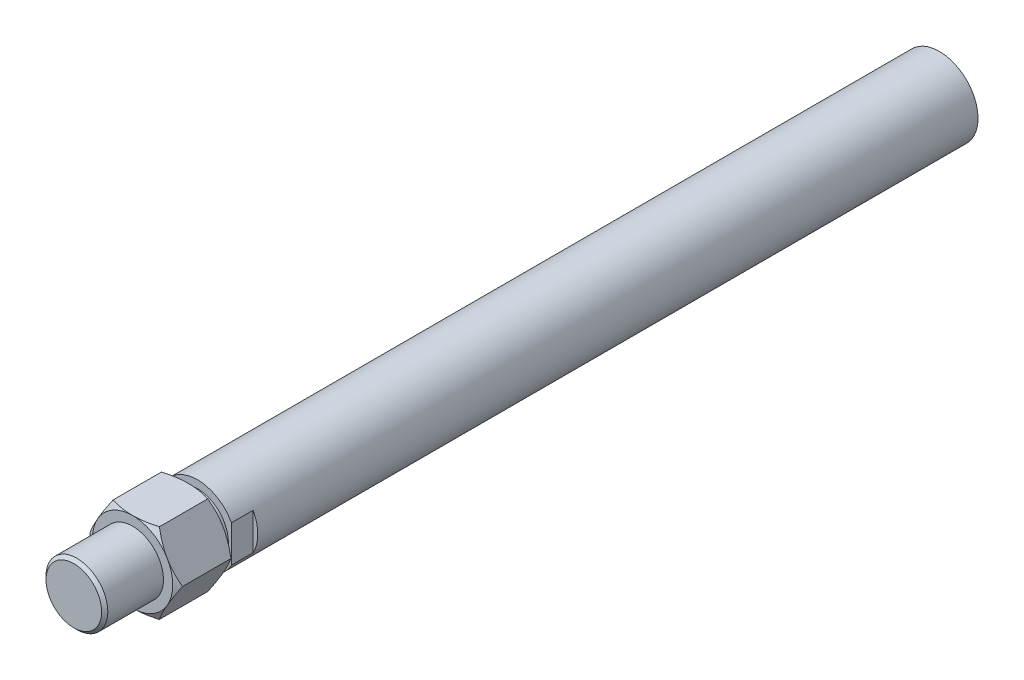
SolidWorks part; units mm, degrees
material "1.4000 (X6Cr13)"
ref_plane "Front Plane" through (0, 0, 0) normal (0, 0, 1) x (1, 0, 0)
ref_plane "Top Plane" through (0, 0, 0) normal (0, 1, 0) x (1, 0, 0)
ref_plane "Right Plane" through (0, 0, 0) normal (1, 0, 0) x (0, 0, -1)
sketch "Sketch1" plane through (0, 0, 0) normal (1, 0, 0) x (0, 0, -1)
  line L0 (0, 0) -> (-318, 0) construction
  line L1 (-243, 23.5) -> (0, 23.5)
  line L2 (0, 23.5) -> (0, -23.5)
  line L3 (0, -23.5) -> (-243, -23.5)
  line L24 (-243, 23.5) -> (-257, 23.5)
  line L25 (-257, 23.5) -> (-257, -23.5)
  line L26 (-257, 22.5208) -> (-264, 22.5208)
  line L27 (-264, 22.5208) -> (-264, -22.5208)
  line L28 (-264, 12.5) -> (-278, 12.5)
  line L29 (-278, 12.5) -> (-278, 10)
  line L30 (-278, 10) -> (-281, 10)
  line L31 (-318, 10) -> (-318, -10)
  line L32 (-278, -10) -> (-281, -10)
  line L33 (-264, -12.5) -> (-278, -12.5)
  line L34 (-257, -22.5208) -> (-264, -22.5208)
  line L35 (-243, -23.5) -> (-257, -23.5)
  line L38 (-299, 10) -> (-299, 15)
  line L39 (-299, 15) -> (-281, 15)
  line L40 (-281, 15) -> (-281, 10)
  line L41 (-281, -15) -> (-281, -10)
  line L42 (-299, -10) -> (-299, -15)
  line L43 (-299, -15) -> (-281, -15)
  line L44 (-299, 10) -> (-318, 10)
  line L45 (-299, -10) -> (-318, -10)
  line L46 (-278, -10) -> (-278, -12.5)
  point P4 (-60, 23.5)
  point P5 (-50, 23.5)
  point P6 (-38, 23.5)
  point P42 (-318, 0)
  point P44 (-318, 0)
  point P46 (-264, 0)
  point P48 (-257, 0)
  dimension "K" = 38
  dimension "RD" = 47
  dimension "KK" = 20
  dimension "VF" = 21
  dimension "WF" = 35
  dimension "D8" = 14
  dimension "S2" = 50
  dimension "S1" = 10
  dimension "A" = 40
  dimension "D14" = 45.0417
  dimension "螺母厚度" = 18
  dimension "D16" = 3
  dimension "螺母外径" = 30
  dimension "MM" = 25
  dimension "L1" = 183
sketch "Sketch3" plane through (0, 0, 0) normal (1, 0, 0) x (0, 0, -1)
  line L0 (-299, 10) -> (-318, 10) construction
  line L1 (-299, 15) -> (-281, 15) construction
  line L2 (-299, 10) -> (-299, 15) construction
  line L3 (-318, 10) -> (-318, -10) construction
  line L11 (-278, 10) -> (-281, 10) construction
  line L12 (-281, 15) -> (-281, 10) construction
  line L13 (-278, 12.5) -> (-278, 10) construction
  line L14 (-264, 12.5) -> (-278, 12.5) construction
  line L17 (-299, 10) -> (-318, 10)
  line L18 (-299, 15) -> (-281, 15)
  line L19 (-299, 10) -> (-299, 15)
  line L20 (-318, 10) -> (-318, 0)
  line L21 (-318, 0) -> (-38, 0)
  line L28 (-278, 10) -> (-281, 10)
  line L29 (-281, 15) -> (-281, 10)
  line L30 (-278, 12.5) -> (-278, 10)
  line L31 (-38, 12.5) -> (-278, 12.5)
  line L34 (-38, 12.5) -> (-38, 0)
  line L36 (0, 0) -> (-318, 0) construction
revolve "Revolve1" add sketch "Sketch3" angle 360 about L21
cosmetic thread "Cosmetic Thread1" parameters "D1"=38, "D2"=17
sketch "Sketch5" plane through (0, 0, 299) normal (0, 0, 1) x (1, 0, 0)
  line L0 (0, 0) -> (15, 0) construction
  line L1 (7.5, 12.9904) -> (-7.5, 12.9904)
  line L2 (-7.5, 12.9904) -> (-15, 0)
  line L3 (-15, 0) -> (-7.5, -12.9904)
  line L4 (-7.5, -12.9904) -> (7.5, -12.9904)
  line L5 (7.5, -12.9904) -> (15, 0)
  line L6 (15, 0) -> (7.5, 12.9904)
  circle A0 centre (0, 0) radius 12.9904 construction
  circle A1 centre (0, 0) radius 15 construction
extrude "Cut-Extrude1" cut sketch "Sketch5" against normal up to surface (18 mm away) flip side to cut up to face at (0, -10, 281)
sketch "Sketch6" plane through (0, 0, 299) normal (0, 0, 1) x (1, 0, 0)
  line L0 (7.5, 12.9904) -> (-7.5, 12.9904) construction
  circle A0 centre (0, 0) radius 12.9904
extrude "Cut-Extrude2" cut sketch "Sketch6" against normal blind 10 draft 60 flip side to cut
sketch "Sketch7" plane through (0, 0, 281) normal (0, 0, -1) x (-1, 0, 0)
  line L0 (7.5, 12.9904) -> (15, 0) construction
  circle A0 centre (0, 0) radius 12.9904
extrude "Cut-Extrude3" cut sketch "Sketch7" against normal blind 10 draft 60 flip side to cut
sketch "Sketch8" plane through (0, 0, 38) normal (0, 0, -1) x (-1, 0, 0)
  point P0 (0, 0)
sketch "Sketch9" plane through (0, 0, 278) normal (0, 0, 1) x (1, 0, 0)
  line L0 (0, 12.9904) -> (0, -12.9904) construction
  line L1 (-11, 12.9904) -> (-11, -12.9904)
  line L2 (11, 12.9904) -> (11, -12.9904)
  line L3 (-11, 12.9904) -> (-33, 12.9904)
  line L4 (-33, 12.9904) -> (-33, -12.9904)
  line L5 (-33, -12.9904) -> (-11, -12.9904)
  line L6 (33, -12.9904) -> (11, -12.9904)
  line L7 (33, 12.9904) -> (33, -12.9904)
  line L8 (11, 12.9904) -> (33, 12.9904)
  arc A0 (0, 12.9904) -> (-11.25, 6.4952) centre (0, 0) ccw construction
  arc A1 (0, -12.9904) -> (11.25, -6.4952) centre (0, 0) ccw construction
  dimension "D" = 22
  dimension "D2" = 22
extrude "Cut-Extrude4" cut sketch "Sketch9" against normal blind 7
chamfer "Chamfer1" distance 1 angle 45 1 edges at (0, -10, 318)
